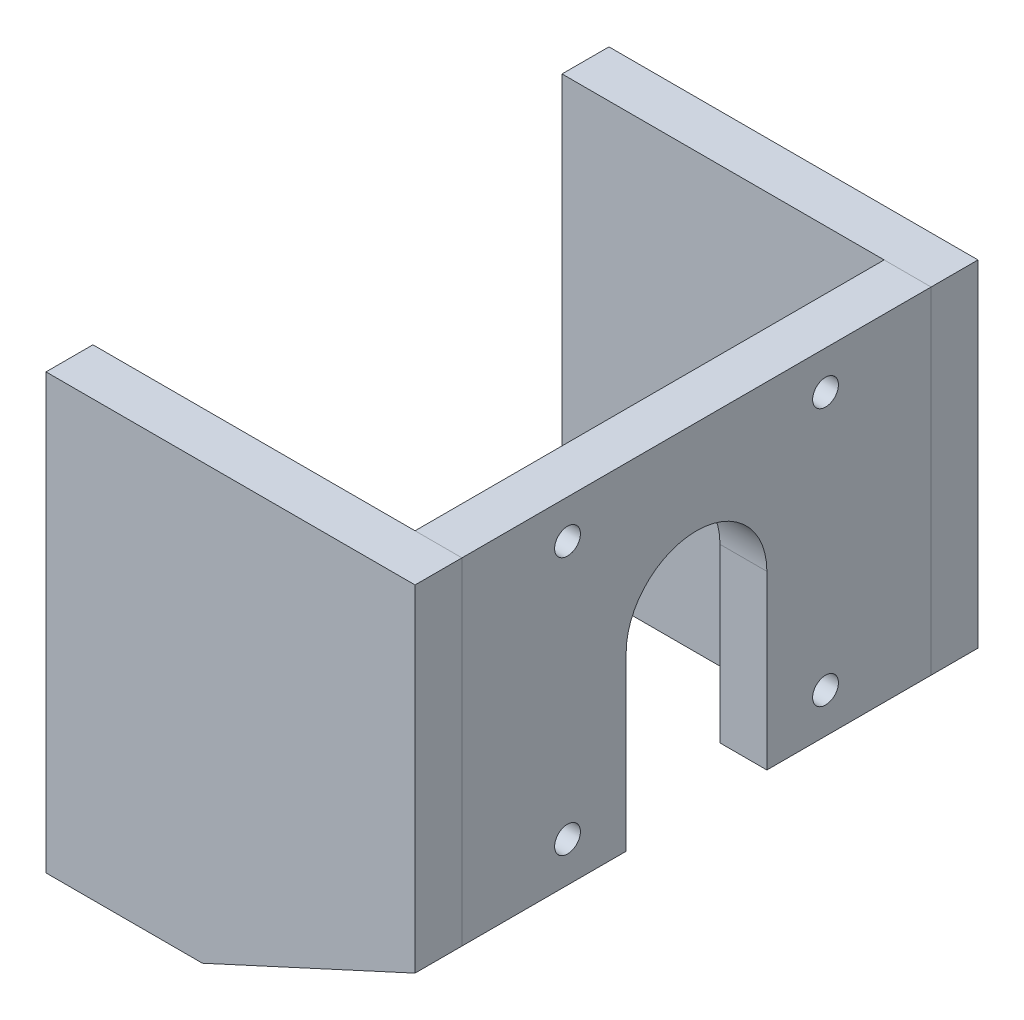
from build123d import *

# Parameters (mm, degrees)
BOSS_EXTRUDE1_DEPTH = 30
BOSS_EXTRUDE2_START = 118
SKETCH5_R           = 8.25
BOSS_EXTRUDE2_DEPTH = 30


with BuildPart() as part:
    # Sketch1 → Boss-Extrude1 (new body)
    with BuildSketch(Plane.XY):
        Polygon((-118, 138.75), (-118, -138.75), (-18, -138.75), (118, -76.25), (118, 138.75), align=None)
    extrude(amount=BOSS_EXTRUDE1_DEPTH)


with BuildPart() as body_2:
    # Mirror2: mirrored copy
    add(part.part.mirror(Plane(origin=(0, 0, -150), x_dir=(1, 0, 0), z_dir=(0, 0, -1))))


with BuildPart() as body_3:
    # Sketch5 → Boss-Extrude2 (new body)
    with BuildSketch(Plane(origin=(0, 0, 0), x_dir=(0, 0, -1), z_dir=(1, 0, 0)).offset(BOSS_EXTRUDE2_START)):
        with BuildLine():
            Line((195, 33.75), (195, -76.25))
            Line((195, -76.25), (300, -76.25))
            Line((300, -76.25), (300, 138.75))
            Line((300, 138.75), (150, 138.75))
            Line((150, 138.75), (0, 138.75))
            Line((0, 138.75), (0, -76.25))
            Line((0, -76.25), (105, -76.25))
            Line((105, -76.25), (105, 33.75))
            ThreePointArc((105, 33.75), (150, 78.75), (195, 33.75))
        make_face()
        with Locations(Location((67.5, 114.25, 0), (0, 0, 180))):
            Circle(SKETCH5_R, mode=Mode.SUBTRACT)
        with Locations(Location((232.5, 114.25, 0), (0, 0, 180))):
            Circle(SKETCH5_R, mode=Mode.SUBTRACT)
        with Locations(Location((232.5, -50.75, 0), (0, 0, 180))):
            Circle(SKETCH5_R, mode=Mode.SUBTRACT)
        with Locations(Location((67.5, -50.75, 0), (0, 0, 180))):
            Circle(SKETCH5_R, mode=Mode.SUBTRACT)
    extrude(amount=-BOSS_EXTRUDE2_DEPTH)


solid = Compound([part.part, body_2.part, body_3.part])
